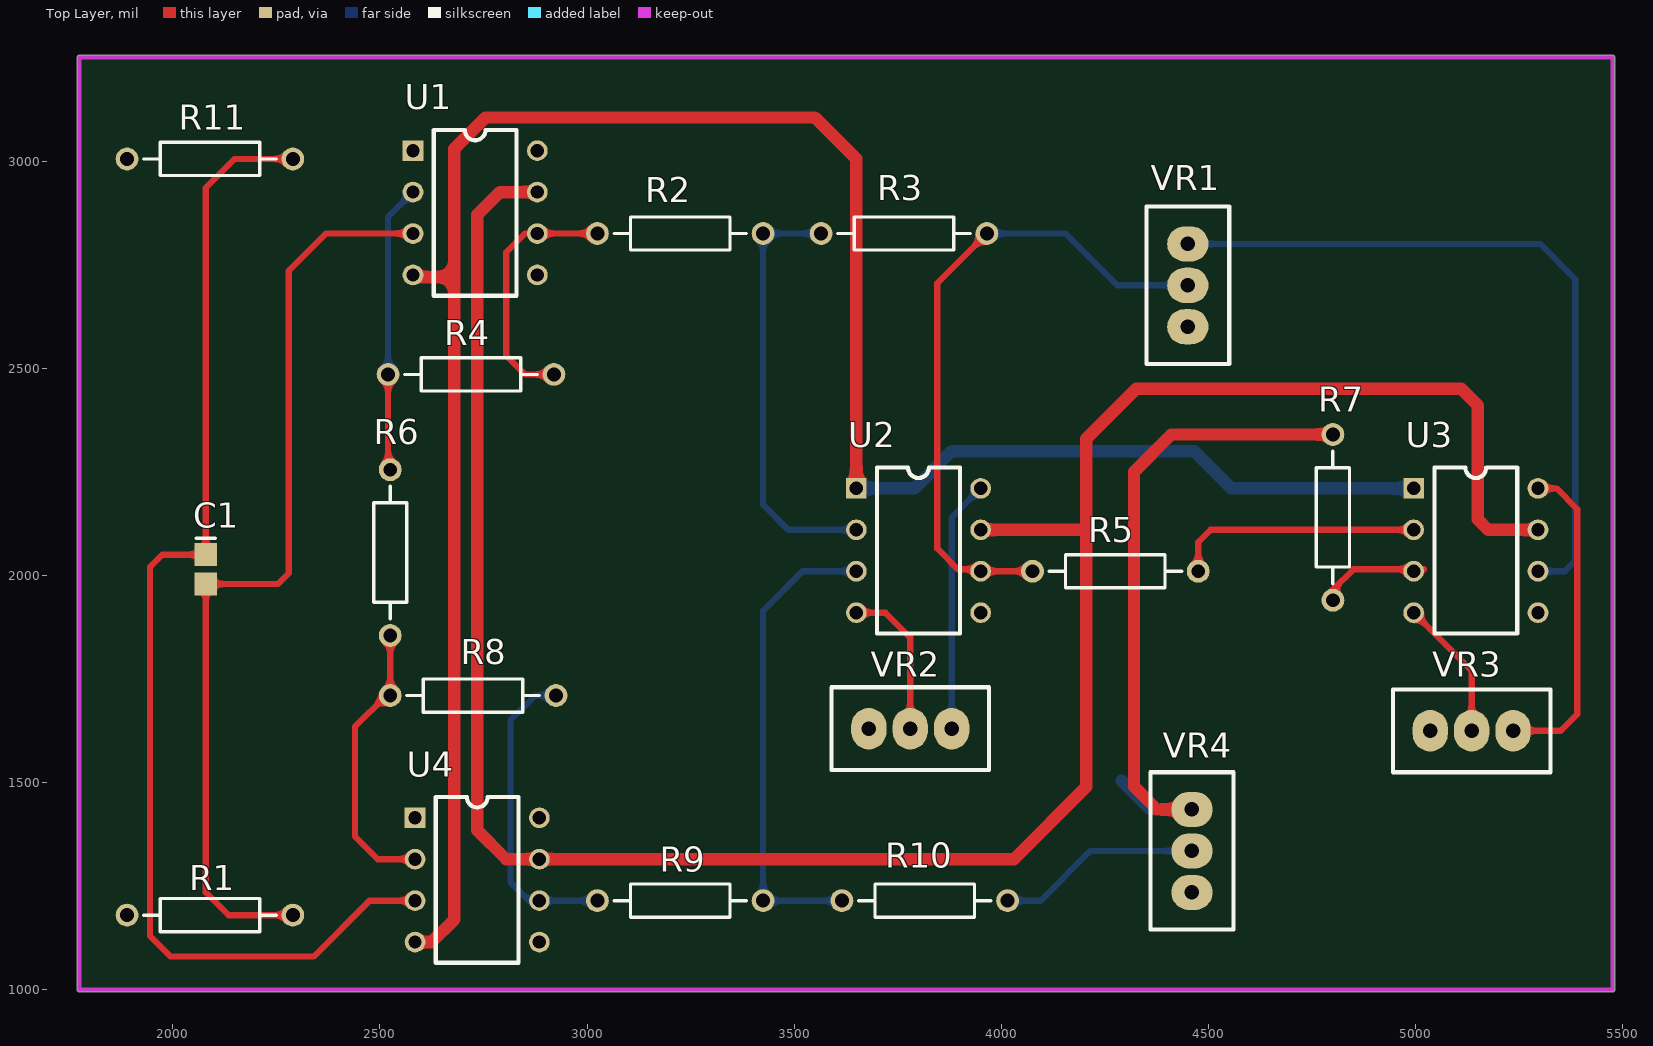
[diagram p0: Top Layer view]
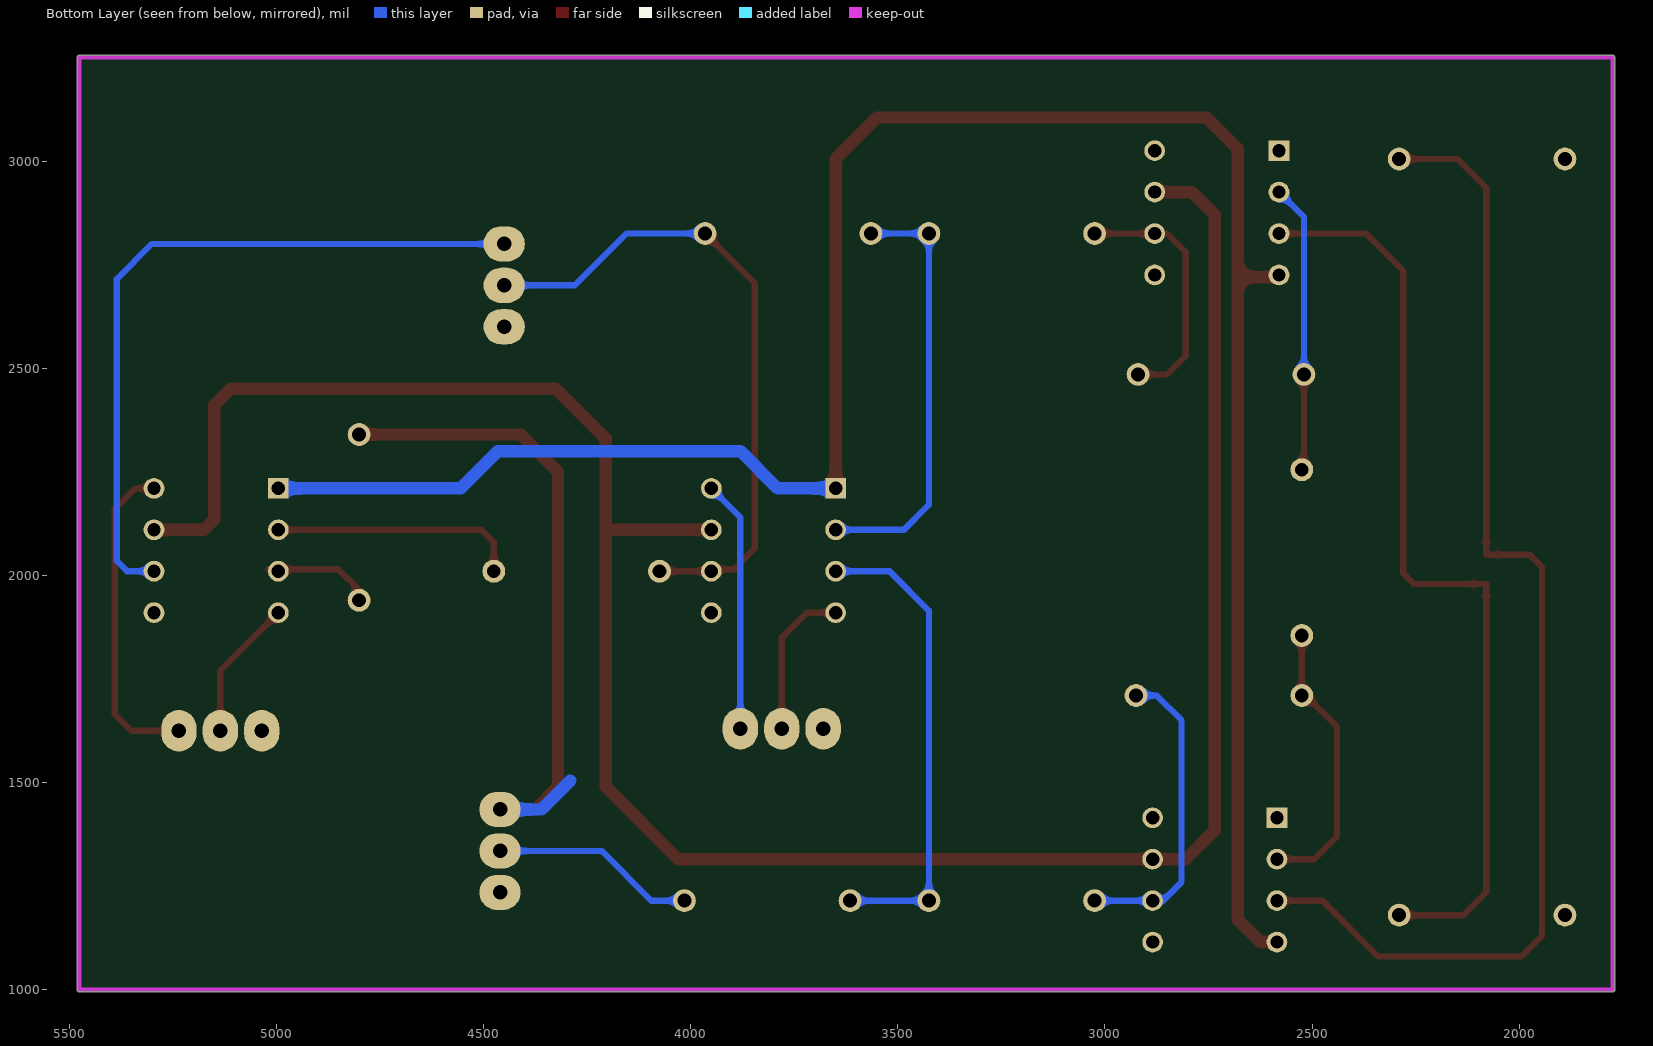
[diagram p1: Bottom Layer view, seen from below]
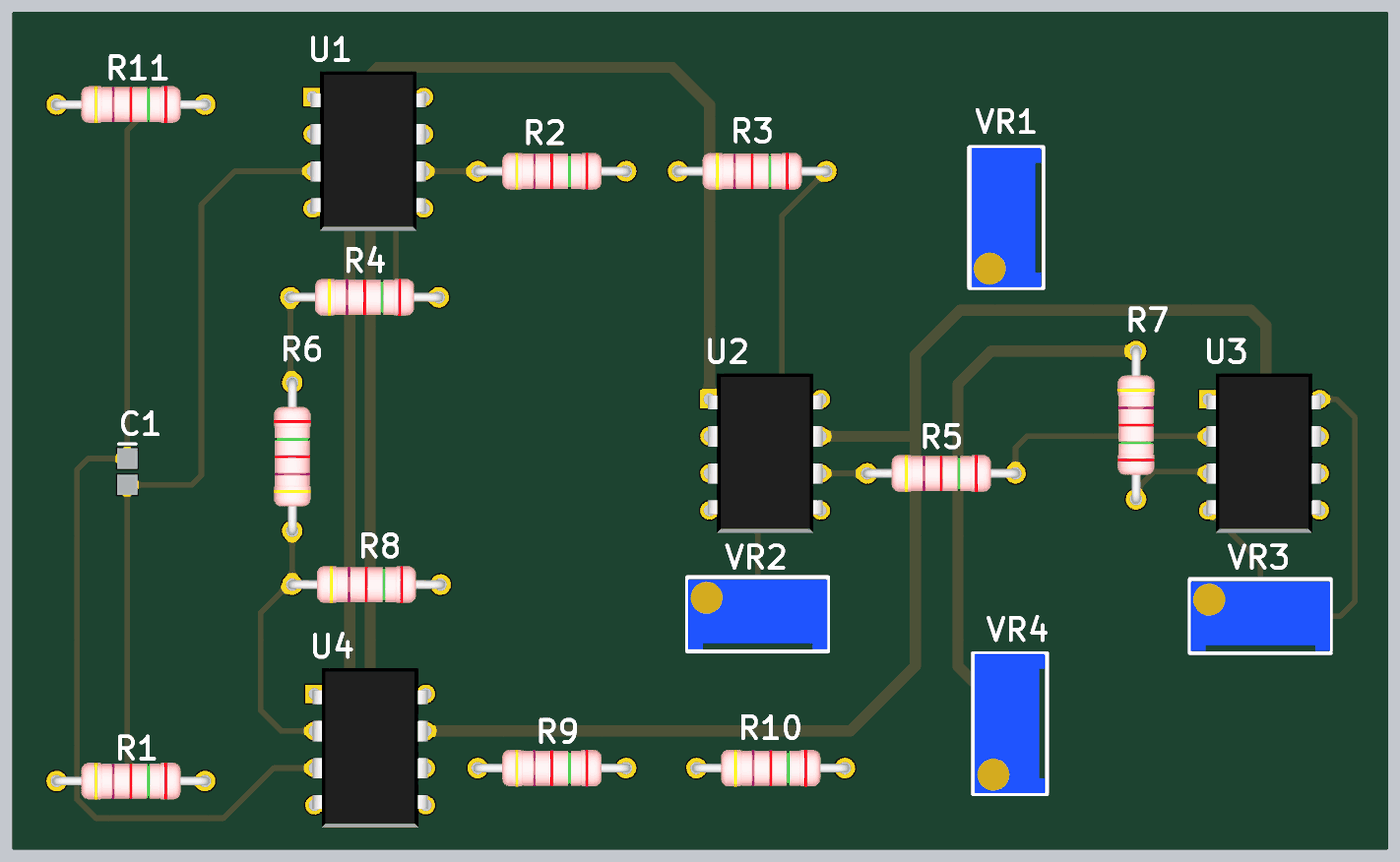
[diagram p2: 3D render of the assembled board from above, using the file's embedded part models]
# Altium PCB MISC89336.PcbDoc
Units mil, origin at the board's own origin, x right, y up, seen from the top; angles counter-clockwise.
Board outline 3710.03 x 2260.03 mil, 2 copper layers (Top Layer, Bottom Layer); 20 components, 20 nets, 68 pads, 0 vias.

## Layer stack, top to bottom (the 12.6 mil dielectric is the usual default, probably not edited)
Top Solder: solder mask 0.4, Solder Resist, Dk 3.5
Top Layer: signal copper 1.4
Dielectric 1: dielectric 12.6, FR-4, Dk 4.8
Bottom Layer: signal copper 1.4
Bottom Solder: solder mask 0.4, Solder Resist, Dk 3.5

## Board outline
1769.98,1000 ccw(c1775,1000) 1775,994.99 5475,994.99 ccw(c5475,1000) 5480.02,1000 5480.02,3250 ccw(c5475,3250) 5475,3255.01 1775,3255.01 ccw(c1775,3250) 1769.98,3250

## Design rules (kind name [scope] priority, off if disabled: settings)
Clearance [All] p1: gap=10
HoleSize [All] p1: absolutevalues=TRUE maxlimit=9999 minlimit=1 maxpercent=80.000 minpercent=20.000
MinimumSolderMaskSliver [All] p1: minsoldermaskwidth=0
PolygonConnect [All] p1: connectstyle=Relief reliefconductorwidth=10 reliefentries=4 polygonreliefangle="90 Angle" airgapwidth=10
RoutingVias [All] p1: holewidth=28 width=50 viastyle="Through Hole" minholewidth=28 minwidth=50 maxholewidth=28 maxwidth=50
SilkToSilkClearance [All] p1: silktosilkclearance=0
SilkToSolderMaskClearance [IsPad] p1: minsilkscreentomaskgap=0 clearancetoexposedcopper=TRUE
SolderMaskExpansion [All] p1: expansion=4
Width [All] p1: maxlimit=30 minlimit=10 preferedwidth=10
26 further rules are at their usual default settings.

## Components (designator, comment, footprint, x,y, rotation, side; value= is the part's Value field where it differs from the comment)
C1 "0.05UF" C2512 2080,2014.57 r270 top
R1 "200K" AXIAL0.4 1760,1140 r0 top
R2 "10K" AXIAL0.4 2895,2785 r0 top
R3 "39K" AXIAL0.4 3435,2785 r0 top
R4 "100K" AXIAL0.4 2390,2445 r0 top
R5 "10K" AXIAL0.4 3945,1970 r0 top
R6 "51K" AXIAL0.4 2565,1725 r90 top
R7 "10K" AXIAL0.4 4760,2470 r270 top
R8 "100K" AXIAL0.4 2395,1670 r0 top
R9 "10K" AXIAL0.4 2895,1175 r0 top
R10 "91K" AXIAL0.4 3485,1175 r0 top
R11 "200K" AXIAL0.4 1760,2965 r0 top
U1 "OP07AH" DIP8 2580,3025 r0 top
U2 "OP07AH" DIP8 3650,2210 r0 top
U3 "OP07AH" DIP8 4995,2210 r0 top
U4 "OP07AH" DIP8 2585,1415 r0 top
VR1 "100K" 3296W 4450,2700 r270 top
VR2 "20K" 3296W 3780,1630 r180 top
VR3 "20K" 3296W 5135,1625 r180 top
VR4 "20K" 3296W 4460,1335 r270 top

## Footprints (in the part's own frame and the unit in brackets; to place one, negate y for a bottom-side part, rotate by r counter-clockwise, add the part's x,y. Pads: shape width x height; smd on the part's side, far side on the other; paste and mask are expansions set on the pad)
3296W [mil]
  oval 85x100 hole 35: 1(-100,0) 2(0,0) 3(100,0)
  silkscreen extent -190,-100 190,100, body extent -188,-94 188,94, height 455
AXIAL0.4 [mm] "1/4W/1/2W"
  round 1.4 hole 0.85: 1(3.302,1.016) 2(13.462,1.016)
  silkscreen extent 4.32,0 12.45,2.03, body extent 3,-0.24 13.76,2.28, height 2.63
C2512 [mm] "Chip Capacitor, Body 2.54x1.27mm, IPC High Density"
  rect 1.4x1.4 smd: 1(-0.9,0) 2(0.9,0)
  silkscreen extent -1.9,-0.6 -1.9,0.6, body extent -1.45,-0.82 1.45,0.82, height 1.3
DIP8 [mil]
  rect 50x50 hole 32: 1(0,0)
  round 50 hole 32: 2(0,-100) 3(0,-200) 4(0,-300) 5(300,-300) 6(300,-200) 7(300,-100) 8(300,0)
  silkscreen extent 50,-350 250,50, body extent -5,-360 305,70, height 200

## Part data
C1: library part "Cap Semi", "Capacitor (Semiconductor SIM Model)"
R1 R2 R3 R4 R5 R6 R7 R8 R9 R10 R11: library part RES
U1 U2 U3 U4: library part ADOP07AH, "Ultra-Low Offset Voltage Operational Amplifier"
VR1 VR2 VR3 VR4: library part RESVR

## Nets (pads, with @x,y where several pads share a name; then routed paths per layer and width w, separated by ;. In a path a pad name is that pad's centre, name@x,y a point inside that pad or via, vN(x,y) a via of type N, cw(c..) or ccw(c..) an arc to the next point about the centre after c; other vN are vias at no path point)
+15V: U1.4 U2.1 U3.1 U4.4 | length 5336.9
  Top Layer w30: U1.4 2585,2720 2680,2720 ; U4.4 2625,1115 2680,1170 2680,2720 ; U2.1 3650,3005 3550,3105 2755,3105 2680,3030 2680,2720
  Bottom Layer w30: U2.1 3790,2210 3880,2300 4465,2300 4555,2210 U3.1
-15V: U1.7 U2.7 U3.7 U4.7 | length 5763
  Top Layer w30: U1.7 2790,2925 2735,2870 2735,1385 2805,1315 U4.7 4030,1315 4205,1490 4205,2115 ; U2.7 4200,2110 4205,2115 ; U3.7 5175,2110 5150,2135 5150,2410 5110,2450 4325,2450 4205,2330 4205,2115
GND: R7.1 VR4.1 | length 1639.1
  Top Layer w30: VR4.1 4375,1435 4320,1490 4320,2250 4410,2340 R7.1
  Bottom Layer w30: 4290,1505 4360,1435 VR4.1
NetC1_1: C1.1 R11.2 U4.3 | length 2878.1
  Top Layer w15: R11.2 2150,3005 2080,2935 C1.1 1975,2050 1945,2020 1945,1130 1995,1080 2340,1080 2475,1215 U4.3
NetC1_2: C1.2 R1.2 U1.3 | length 2254.9
  Top Layer w15: R1.2 2135,1180 2080,1235 C1.2 2254.13,1979.13 2280,2005 2280,2735 2370,2825 U1.3
NetR2_1: R2.1 R4.2 U1.6 | length 622.3
  Top Layer w15: R4.2 2850,2485 2805,2530 2805,2780 2850,2825 U1.6 R2.1
NetR2_2: R2.2 R3.1 U2.2 | length 1044.9
  Bottom Layer w15: R3.1 R2.2 3425,2170 3485,2110 U2.2
NetR3_2: R3.2 R5.1 U2.6 VR1.2 | length 1599.3
  Top Layer w15: R3.2 3845,2705 3845,2065 3895,2015 3945,2015 U2.6 R5.1
  Bottom Layer w15: R3.2 4155,2825 4280,2700 VR1.2
NetR4_1: R4.1 R6.2 U1.2 | length 696.9
  Top Layer w15: R4.1 2520,2260 R6.2
  Bottom Layer w15: R4.1 2520,2865 U1.2
NetR5_2: R5.2 U3.2 | length 602.4
  Top Layer w15: R5.2 4475,2080 4505,2110 U3.2
NetR6_1: R6.1 R8.1 U4.2 | length 693.8
  Top Layer w15: R6.1 R8.1 2515,1710 2440,1635 2440,1370 2495,1315 U4.2
NetR7_2: R7.2 U3.3 | length 292.8
  Top Layer w15: R7.2 4800,1965 4850,2015 5020,2015 5015,2010 U3.3
NetR8_2: R8.2 R9.1 U4.6 | length 753.5
  Bottom Layer w15: R8.2 2875,1710 2815,1650 2815,1260 2860,1215 U4.6 R9.1
NetR9_2: R9.2 R10.1 U2.3 | length 1154.4
  Bottom Layer w15: R10.1 R9.2 3425,1915 3520,2010 U2.3
NetR10_2: R10.2 VR4.2 | length 494.7
  Bottom Layer w15: R10.2 4095,1215 4215,1335 VR4.2
NetU2_4: U2.4 VR2.2 | length 374.9
  Top Layer w15: U2.4 3720,1910 3780,1850 VR2.2
NetU2_8: U2.8 VR2.1 | length 609
  Bottom Layer w15: VR2.1 3880,2140 U2.8
NetU3_4: U3.4 VR3.2 | length 343
  Top Layer w15: U3.4 5135,1770 VR3.2
NetU3_6: U3.6 VR1.1 | length 1750.6
  Bottom Layer w15: VR1.1 5300,2800 5385,2715 5385,2035 5360,2010 U3.6
NetU3_8: U3.8 VR3.1 | length 782.3
  Top Layer w15: VR3.1 5350,1625 5390,1665 5390,2160 5340,2210 U3.8
pads on no net: R1.1 R11.1 U1.1 U1.5 U1.8 U2.5 U3.5 U4.1 U4.5 U4.8 VR1.3 VR2.3 VR3.3 VR4.3

## Keep-outs
Keep-Out Layer:
  lines w10: 5475,2850 5475,3250 1775,3250 1775,1000 5475,1000 5475,2950